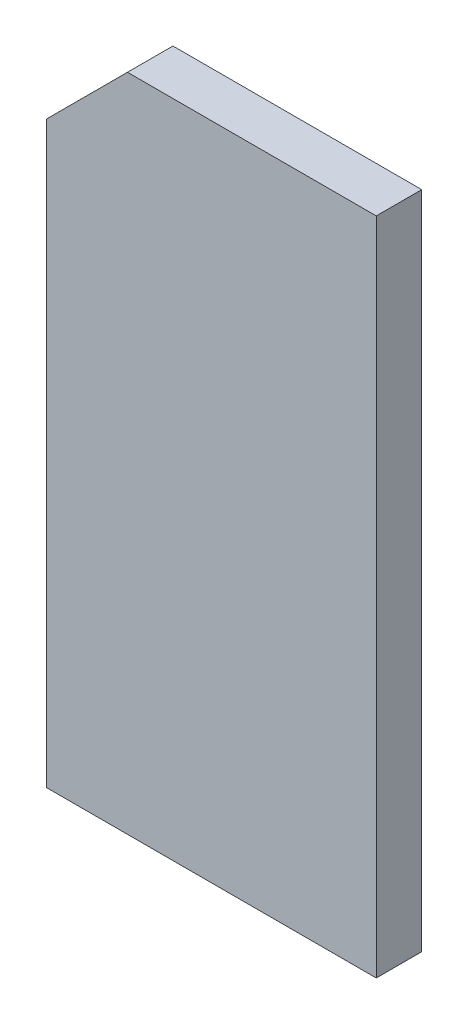
SolidWorks part; units mm, degrees
material "Q235B"
ref_plane "Front Plane" through (0, 0, 0) normal (0, 0, 1) x (1, 0, 0)
ref_plane "Top Plane" through (0, 0, 0) normal (0, 1, 0) x (1, 0, 0)
ref_plane "Right Plane" through (0, 0, 0) normal (1, 0, 0) x (0, 0, -1)
sketch "Sketch1" plane through (0, 0, 0) normal (0, 0, 1) x (1, 0, 0)
  line L1 (0, 0) -> (101.6, 0)
  line L2 (0, 0) -> (0, 203.2)
  line L3 (0, 203.2) -> (101.6, 203.2)
  line L4 (101.6, 0) -> (101.6, 203.2)
  dimension "D1" = 203.2
  dimension "D2" = 101.6
extrude "Extrude1" add sketch "Sketch1" along normal mid plane 14
chamfer "Chamfer1" distance 25 angle 45 1 edges at (0, 203.2, 0)
